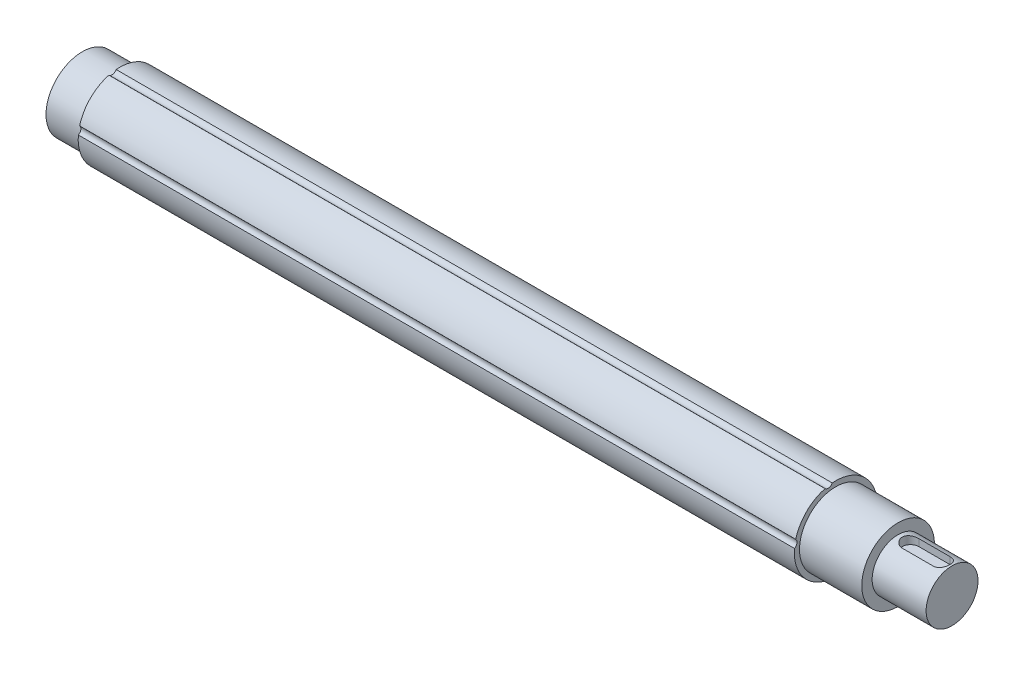
from build123d import *

# Parameters (mm, degrees)
CUT_EXTRUDE_1_DEPTH      = 205.5
CUT_EXTRUDE_1_DEPTH_BACK = 205.5
SKETCH_2_R               = 40
SKETCH_3_OUTSIDE_W       = 124.974
SKETCH_3_OUTSIDE_H       = 124.974
SKETCH_3_OUTSIDE_R       = 17.5
CUT_EXTRUDE_2_DEPTH      = 18
SKETCH_4_OUTSIDE_W       = 124.974
SKETCH_4_OUTSIDE_H       = 124.974
SKETCH_4_OUTSIDE_R       = 12.5
CUT_EXTRUDE_3_DEPTH      = 18
SKETCH_5_OUTSIDE_W       = 124.974
SKETCH_5_OUTSIDE_H       = 124.974
SKETCH_5_OUTSIDE_R       = 17.5
CUT_EXTRUDE_4_DEPTH      = 30
EXTRUDE_START            = 8
SKETCH_7_R               = 12.5
EXTRUDE_1_DEPTH          = 8
CUT_EXTRUDE_5_DEPTH      = 4


with BuildPart() as part:
    # 草图1 → 旋转1 (revolve)
    with BuildSketch(Plane.XY, mode=Mode.PRIVATE) as revolve_1_sk:
        Polygon((-205.5, 0), (-205.5, 19), (-204.5, 20), (204.5, 20), (205.5, 19), (205.5, 0), align=None)
    revolve(revolve_1_sk.sketch.rotate(Axis((205.5, 0, 0), (-1, 0, 0)), 270), axis=Axis((205.5, 0, 0), (-1, 0, 0)))

    # 草图2 → 切除-拉伸1 (cut, two sides: drawn at the far end of the back side and taken through both)
    with BuildSketch(Plane(origin=(0, 0, 0), x_dir=(0, 0, -1), z_dir=(1, 0, 0)).offset(-CUT_EXTRUDE_1_DEPTH_BACK)):
        Circle(SKETCH_2_R)
        with BuildLine():
            ThreePointArc((-19.926297295, 1.715423015), (-14.142135624, -14.142135624), (1.715423015, -19.926297295))
            ThreePointArc((1.715423015, -19.926297295), (3.302788339, -18.731043462), (5.203224708, -19.311303753))
            ThreePointArc((5.203224708, -19.311303753), (14.142135624, -14.142135624), (19.311303753, -5.203224708))
            ThreePointArc((19.311303753, -5.203224708), (18.731043462, -3.302788339), (19.926297295, -1.715423015))
            ThreePointArc((19.926297295, -1.715423015), (14.142135624, 14.142135624), (-1.715423015, 19.926297295))
            ThreePointArc((-1.715423015, 19.926297295), (-3.302788339, 18.731043462), (-5.203224708, 19.311303753))
            ThreePointArc((-5.203224708, 19.311303753), (-14.142135624, 14.142135624), (-19.311303753, 5.203224708))
            ThreePointArc((-19.311303753, 5.203224708), (-18.731043462, 3.302788339), (-19.926297295, 1.715423015))
        make_face(mode=Mode.SUBTRACT)
    extrude(amount=CUT_EXTRUDE_1_DEPTH + CUT_EXTRUDE_1_DEPTH_BACK, mode=Mode.SUBTRACT)

    # 草图3 outside → 切除-拉伸2 (cut)
    with BuildSketch(Plane.ZY.offset(205.5)):
        Rectangle(SKETCH_3_OUTSIDE_W, SKETCH_3_OUTSIDE_H)
        Circle(SKETCH_3_OUTSIDE_R, mode=Mode.SUBTRACT)
    extrude(amount=-CUT_EXTRUDE_2_DEPTH, mode=Mode.SUBTRACT)

    # 草图4 outside → 切除-拉伸3 (cut)
    with BuildSketch(Plane(origin=(205.5, 0, 0), x_dir=(0, 0, -1), z_dir=(1, 0, 0))):
        Rectangle(SKETCH_4_OUTSIDE_W, SKETCH_4_OUTSIDE_H)
        Circle(SKETCH_4_OUTSIDE_R, mode=Mode.SUBTRACT)
    extrude(amount=-CUT_EXTRUDE_3_DEPTH, mode=Mode.SUBTRACT)

    # 草图5 outside → 切除-拉伸4 (cut)
    with BuildSketch(Plane(origin=(187.5, 0, 0), x_dir=(0, 0, -1), z_dir=(1, 0, 0))):
        Rectangle(SKETCH_5_OUTSIDE_W, SKETCH_5_OUTSIDE_H)
        with Locations(Location((0, 0, 0), (0, 0, 180))):
            Circle(SKETCH_5_OUTSIDE_R, mode=Mode.SUBTRACT)
    extrude(amount=-CUT_EXTRUDE_4_DEPTH, mode=Mode.SUBTRACT)

    # 草图7 → 凸台-拉伸1 (add)
    with BuildSketch(Plane(origin=(205.5, 0, 0), x_dir=(0, 0, -1), z_dir=(1, 0, 0)).offset(EXTRUDE_START)):
        Circle(SKETCH_7_R)
    extrude(amount=-EXTRUDE_1_DEPTH)

    # 草图6 → 切除-拉伸5 (cut)
    with BuildSketch(Plane(origin=(0, 12.5, 0), x_dir=(1, 0, 0), z_dir=(0, 1, 0))):
        with BuildLine():
            Line((208.5, -4), (193.5, -4))
            ThreePointArc((193.5, -4), (189.5, 0), (193.5, 4))
            Line((193.5, 4), (208.5, 4))
            ThreePointArc((208.5, 4), (212.5, 0), (208.5, -4))
        make_face()
    extrude(amount=-CUT_EXTRUDE_5_DEPTH, mode=Mode.SUBTRACT)


solid = part.part
